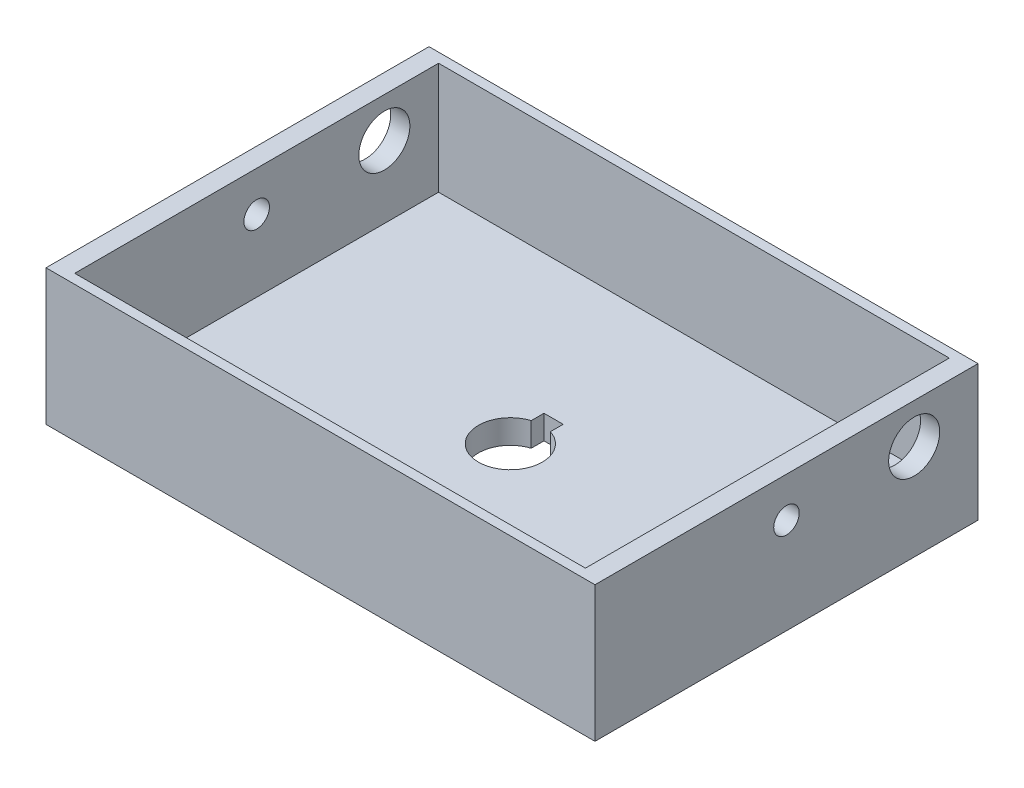
from build123d import *

# Parameters (mm, degrees)
SKETCH_1_W          = 172
SKETCH_1_H          = 42.5
EXTRUDE_2_DEPTH     = 120
CUT_EXTRUDE_1_DEPTH = 35
SKETCH_5_R          = 8
SKETCH_5_R_2        = 4
CUT_EXTRUDE_2_DEPTH = 211.797444244
CUT_EXTRUDE_4_DEPTH = 154.630237909


with BuildPart() as part:
    # 草图1 → 凸台-拉伸2 (new body)
    with BuildSketch(Plane.XY):
        Rectangle(SKETCH_1_W, SKETCH_1_H)
    extrude(amount=EXTRUDE_2_DEPTH)

    # 草图2 → 切除-拉伸1 (cut)
    with BuildSketch(Plane(origin=(0, 21.25, 0), x_dir=(1, 0, 0), z_dir=(0, 1, 0))):
        Polygon((-80, -5), (-80, -3), (80, -3), (80, -5), (80, -117), (-80, -117), align=None)
    extrude(amount=-CUT_EXTRUDE_1_DEPTH, mode=Mode.SUBTRACT)

    # 草图5 → 切除-拉伸2 (cut, through all)
    with BuildSketch(Plane.ZY.offset(86)):
        with Locations((20, 8.75)):
            Circle(SKETCH_5_R)
        with Locations((60, 8.75)):
            Circle(SKETCH_5_R_2)
    extrude(amount=-CUT_EXTRUDE_2_DEPTH, mode=Mode.SUBTRACT)

    # 草图6 → 切除-拉伸4 (cut, through all)
    with BuildSketch(Plane.XZ.offset(21.25)):
        with BuildLine():
            Line((-3.517636002, 50.460607986), (-3.517636002, 46.460607986))
            Line((-3.517636002, 46.460607986), (2.482363998, 46.460607986))
            Line((2.482363998, 46.460607986), (2.482363998, 50.460607986))
            ThreePointArc((2.482363998, 50.460607986), (-0.517636002, 70), (-3.517636002, 50.460607986))
        make_face()
    extrude(amount=-CUT_EXTRUDE_4_DEPTH, mode=Mode.SUBTRACT)


solid = part.part
